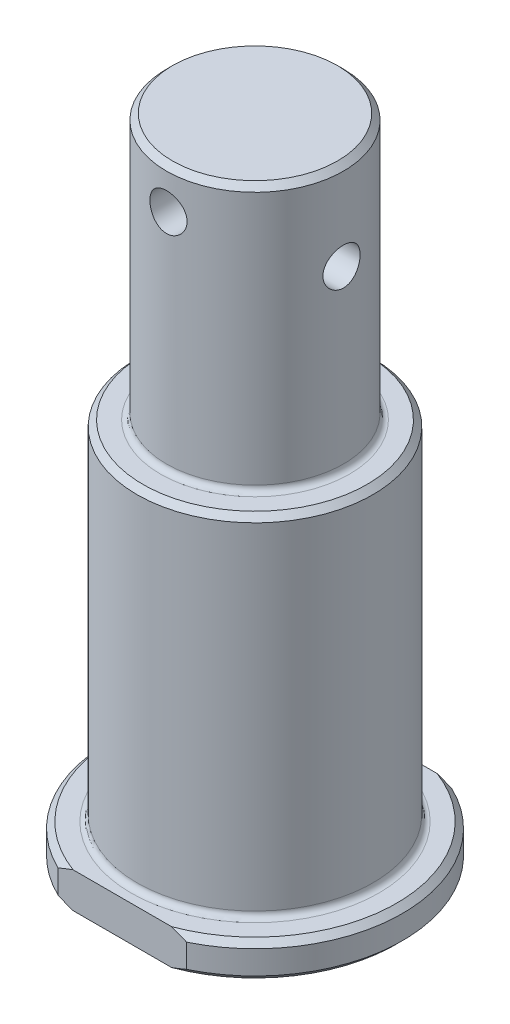
from build123d import *

# Parameters (mm, degrees)
CHAMFER1_SIZE           = 1
FILLET1_R               = 1
SKETCH2_OUTSIDE_W       = 78.154
SKETCH2_OUTSIDE_H       = 78.154
SKETCH2_OUTSIDE_W_2     = 80
SKETCH2_OUTSIDE_H_2     = 45
CUT_EXTRUDE1_DEPTH      = 6
CUT_EXTRUDE2_DEPTH      = 116.027170703
CUT_EXTRUDE2_DEPTH_BACK = 116.027170703
SKETCH3_R               = 3.15
CUT_EXTRUDE3_DEPTH      = 116.027170703
CUT_EXTRUDE3_DEPTH_BACK = 116.027170703
SKETCH4_R               = 3.15


with BuildPart() as part:
    # Sketch1 → Revolve1 (revolve)
    with BuildSketch(Plane.XY, mode=Mode.PRIVATE) as revolve1_sk:
        Polygon((0, 0), (25, 0), (25, 6), (20, 6), (20, 65), (15, 65), (15, 110), (0, 110), align=None)
    revolve(revolve1_sk.sketch.rotate(Axis((0, 0, 0), (0, -1, 0)), 90), axis=Axis((0, 0, 0), (0, -1, 0)))

    # Chamfer1
    chamfer1_edges = [part.edges().sort_by_distance(p)[0] for p in [
        (0, 110, -15),
        (0, 65, -20),
        (0, 6, -25),
        (0, 0, -25),
    ]]
    chamfer(chamfer1_edges, length=CHAMFER1_SIZE)

    # Fillet1
    fillet1_edges = [part.edges().sort_by_distance(p)[0] for p in [
        (0, 65, -15),
        (0, 6, -20),
    ]]
    fillet(fillet1_edges, radius=FILLET1_R)

    # Sketch2 outside → Cut-Extrude1 (cut)
    with BuildSketch(Plane(origin=(0, 0, 0), x_dir=(1, 0, 0), z_dir=(0, 1, 0))):
        Rectangle(SKETCH2_OUTSIDE_W, SKETCH2_OUTSIDE_H)
        Rectangle(SKETCH2_OUTSIDE_W_2, SKETCH2_OUTSIDE_H_2, mode=Mode.SUBTRACT)
    extrude(amount=CUT_EXTRUDE1_DEPTH, mode=Mode.SUBTRACT)

    # Sketch3 → Cut-Extrude2 (cut, two sides: drawn at the far end of the back side and taken through both)
    with BuildSketch(Plane.XY.offset(-CUT_EXTRUDE2_DEPTH_BACK)):
        with Locations(Location((0, 103, 0), (0, 0, 269.99999995))):
            Circle(SKETCH3_R)
    extrude(amount=CUT_EXTRUDE2_DEPTH + CUT_EXTRUDE2_DEPTH_BACK, mode=Mode.SUBTRACT)

    # Sketch4 → Cut-Extrude3 (cut, two sides: drawn at the far end of the back side and taken through both)
    with BuildSketch(Plane(origin=(0, 0, 0), x_dir=(0, 0, -1), z_dir=(1, 0, 0)).offset(-CUT_EXTRUDE3_DEPTH_BACK)):
        with Locations((0, 95)):
            Circle(SKETCH4_R)
    extrude(amount=CUT_EXTRUDE3_DEPTH + CUT_EXTRUDE3_DEPTH_BACK, mode=Mode.SUBTRACT)


solid = part.part
